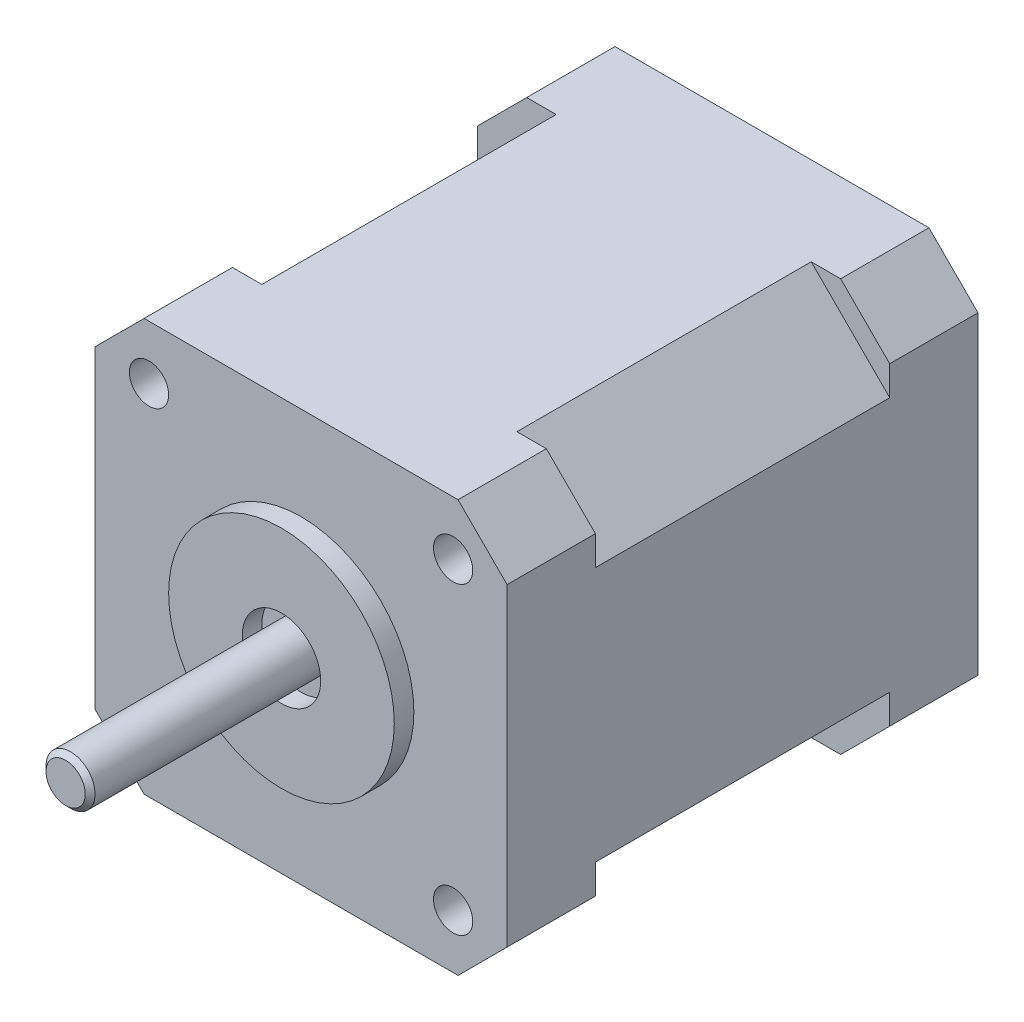
SolidWorks part; units mm, degrees
material "Nickel"
ref_plane "Front Plane" through (0, 0, 0) normal (0, 0, 1) x (1, 0, 0)
ref_plane "Top Plane" through (0, 0, 0) normal (0, 1, 0) x (1, 0, 0)
ref_plane "Right Plane" through (0, 0, 0) normal (1, 0, 0) x (0, 0, -1)
sketch "Sketch1" plane through (0, 0, 0) normal (0, 0, 1) x (1, 0, 0)
  line L1 (21, -21) -> (-21, -21)
  line L2 (21, -21) -> (21, 21)
  line L3 (21, 21) -> (-21, 21)
  line L4 (-21, -21) -> (-21, 21)
  line L5 (21, -21) -> (-21, 21) construction
  line L6 (21, 21) -> (-21, -21) construction
  point P0 (0, 0)
  dimension "D1" = 42
  dimension "D2" = 42
extrude "Boss-Extrude1" add sketch "Sketch1" along normal mid plane 30
chamfer "Chamfer1" distance 8 angle 45 4 edges at (-21, -21, 0) (21, -21, 0) (-21, 21, 0) (21, 21, 0)
sketch "Sketch3" plane through (0, 0, 15) normal (0, 0, 1) x (1, 0, 0)
  line L0 (13, 21) -> (-13, 21) construction
  line L1 (16, -21) -> (-16, -21)
  line L2 (21, -16) -> (21, 16)
  line L3 (16, 21) -> (-16, 21)
  line L4 (-21, -16) -> (-21, 16)
  line L5 (21, -21) -> (-21, 21) construction
  line L6 (21, 21) -> (-21, -21) construction
  line L7 (-21, 13) -> (-21, -13) construction
  line L8 (-16, 21) -> (-21, 16)
  line L9 (21, 16) -> (16, 21)
  line L10 (21, -16) -> (16, -21)
  line L11 (-16, -21) -> (-21, -16)
  point P0 (0, 0)
  dimension "D1" = 5
  dimension "D2" = 45
  dimension "D3" = 5
  dimension "D4" = 45
  dimension "D5" = 5
  dimension "D6" = 45
  dimension "D7" = 5
  dimension "D8" = 45
extrude "Boss-Extrude2" add sketch "Sketch3" along normal blind 9
mirror "Mirror1" about plane through (0, 0, 0) normal (0, 0, 1) of "Boss-Extrude2"
sketch "Sketch4" plane through (0, 0, 24) normal (0, 0, 1) x (1, 0, 0)
  circle A0 centre (0, 0) radius 11.5
  dimension "D1" = 23
extrude "Boss-Extrude3" add sketch "Sketch4" along normal blind 2
sketch "Sketch5" plane through (0, 0, 26) normal (0, 0, 1) x (1, 0, 0)
  circle A0 centre (0, 0) radius 2.5
  dimension "D1" = 5
extrude "Boss-Extrude4" add sketch "Sketch5" along normal blind 22
sketch "Sketch6" plane through (0, 0, 26) normal (0, 0, 1) x (1, 0, 0)
  circle A0 centre (0, 0) radius 4
  circle A1 centre (0, 0) radius 2.5
  circle A2 centre (0, 0) radius 2.5
  dimension "D2" = 8
  dimension "D1" = 0
extrude "Cut-Extrude1" cut sketch "Sketch6" against normal blind 2
chamfer "Chamfer2" distance 0.5 angle 45 1 edges at (2.5, 0, 48)
sketch "Sketch7" plane through (0, 0, 24) normal (0, 0, 1) x (1, 0, 0)
  circle A0 centre (15.5, 15.5) radius 2
  circle A1 centre (15.5, -15.5) radius 2
  circle A2 centre (-15.5, -15.5) radius 2
  circle A3 centre (-15.5, 15.5) radius 2
  point P12 (0, 0)
  dimension "D1" = 4
  dimension "D2" = 15.5
  dimension "D3" = 15.5
  dimension "D4" = 4
extrude "Cut-Extrude2" cut sketch "Sketch7" against normal through all
